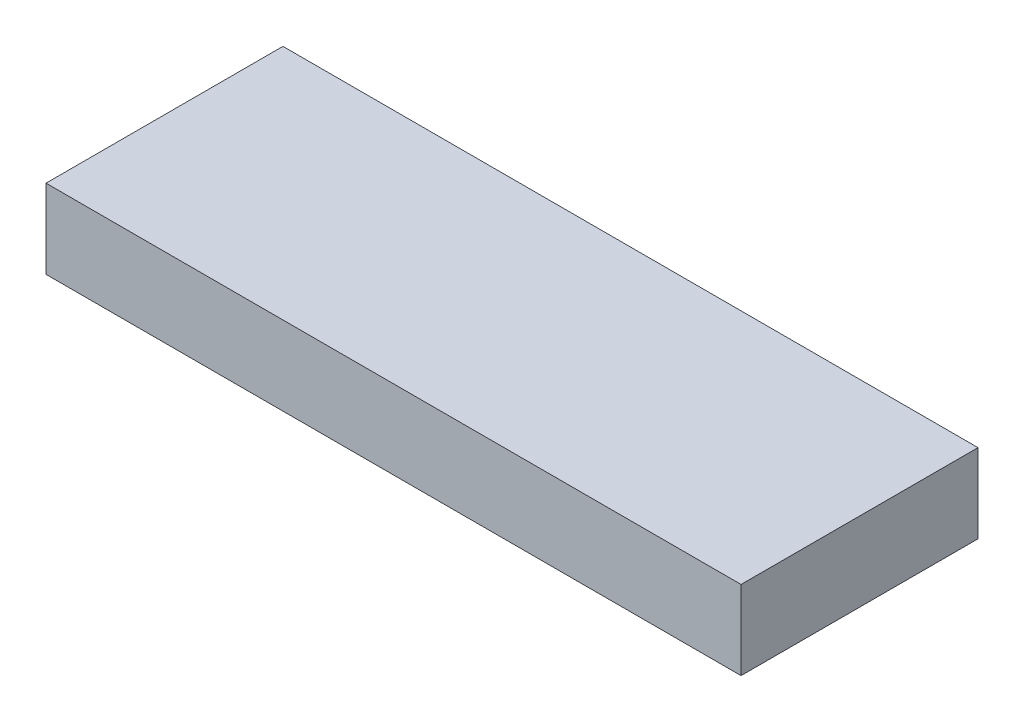
SolidWorks part; units mm, degrees
material "合金钢"
ref_plane "前视基准面" through (0, 0, 0) normal (0, 0, 1) x (1, 0, 0)
ref_plane "上视基准面" through (0, 0, 0) normal (0, 1, 0) x (1, 0, 0)
ref_plane "右视基准面" through (0, 0, 0) normal (1, 0, 0) x (0, 0, -1)
sketch "草图1" plane through (0, 0, 0) normal (0, 1, 0) x (1, 0, 0)
  line L1 (-22, -7.5) -> (22, -7.5)
  line L2 (-22, -7.5) -> (-22, 7.5)
  line L3 (-22, 7.5) -> (22, 7.5)
  line L4 (22, -7.5) -> (22, 7.5)
  line L5 (-22, -7.5) -> (22, 7.5) construction
  line L6 (-22, 7.5) -> (22, -7.5) construction
  point P0 (0, 0)
  dimension "D1" = 44
  dimension "D2" = 15
extrude "凸台-拉伸1" add sketch "草图1" along normal blind 5
